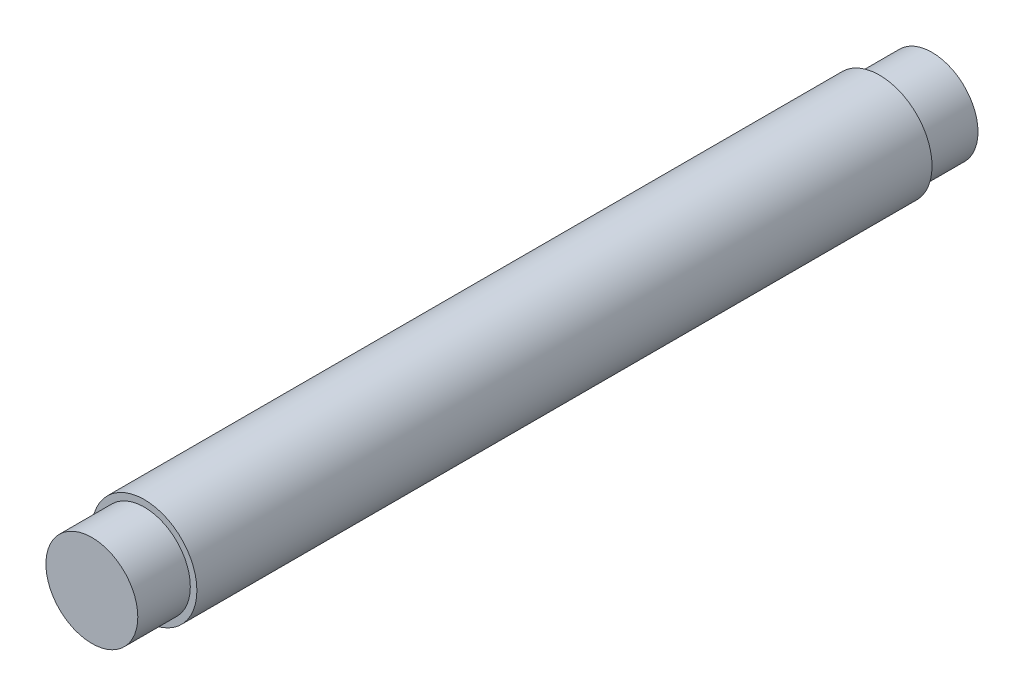
SolidWorks part; units mm, degrees
ref_plane "Front Plane" through (0, 0, 0) normal (0, 0, 1) x (1, 0, 0)
ref_plane "Top Plane" through (0, 0, 0) normal (0, 1, 0) x (1, 0, 0)
ref_plane "Right Plane" through (0, 0, 0) normal (1, 0, 0) x (0, 0, -1)
other "Configuration Table"
sketch "Sketch1" plane through (0, 0, 0) normal (0, 0, 1) x (1, 0, 0)
  circle A0 centre (0, 0) radius 87.5
  dimension "D1" = 175
extrude "Boss-Extrude1" add sketch "Sketch1" along normal mid plane 1600
sketch "Sketch2" plane through (0, 0, 0) normal (0, 0, 1) x (1, 0, 0)
  circle A0 centre (0, 0) radius 100
  dimension "D1" = 200
extrude "Boss-Extrude2" add sketch "Sketch2" along normal mid plane 1400
